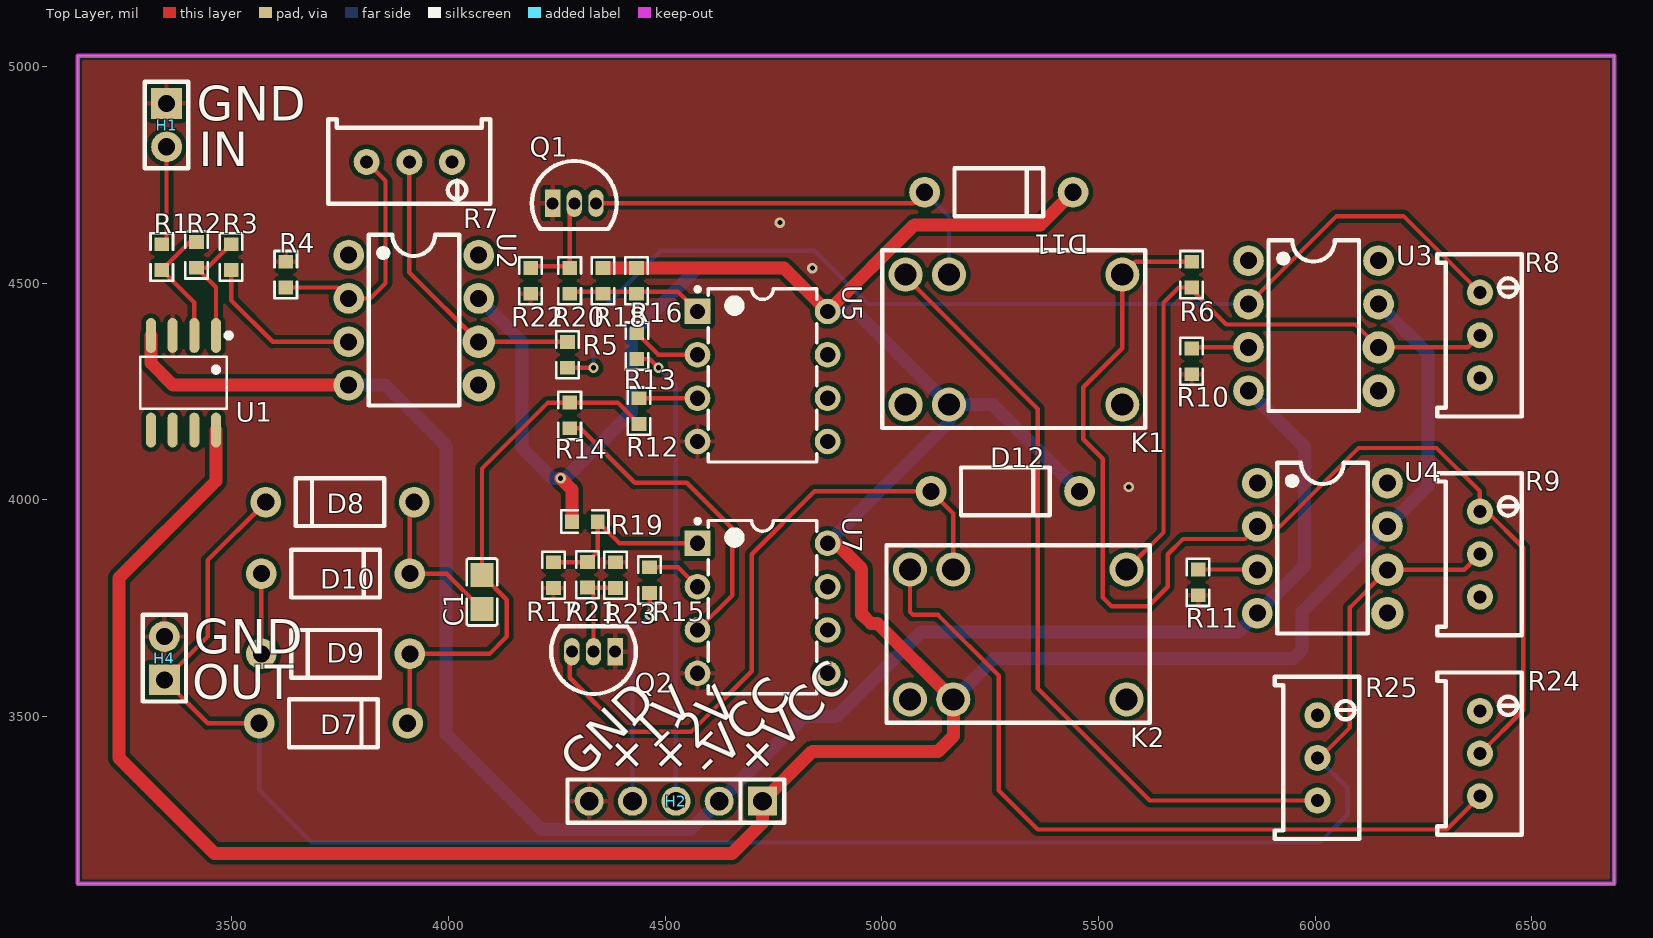
[diagram p0: Top Layer view]
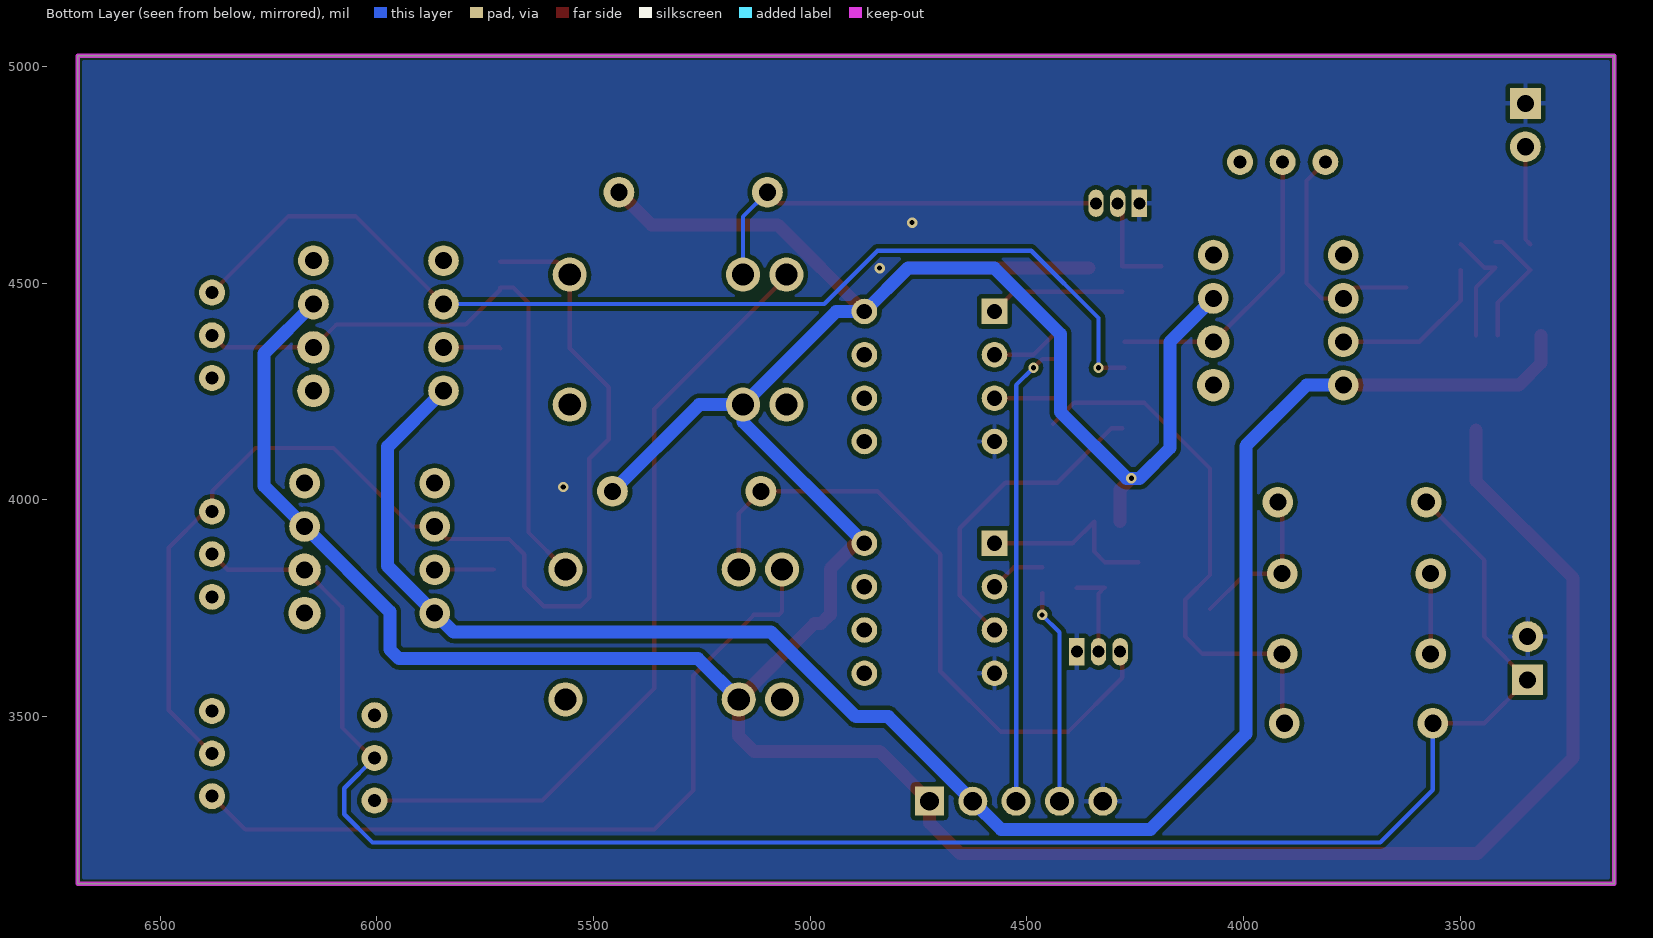
[diagram p1: Bottom Layer view, seen from below]
# Altium PCB MISC51828.pcbdoc
Units mil, origin at the board's own origin, x right, y up, seen from the top; angles counter-clockwise.
Board outline 3545 x 1910 mil, 2 copper layers (Top Layer, Bottom Layer), stack 62.206 mil thick; 45 components, 32 nets, 144 pads, 7 vias.

## Layer stack, top to bottom
Top Solder Mask Layer: solder mask 0.394, Dk 3.3
Top Layer: signal copper 1.379
Dielectric1: surface 59.449, FR4, Dk 4.5
Bottom Layer: signal copper 1.378
Bottom Solder Mask Layer: solder mask 0.394, Dk 3.3

## Board outline
3145,5025 3145,3115 6690,3115 6690,5025

## Design rules (kind name [scope] priority, off if disabled: settings)
BoardOutlineClearance copperThickness2oz_1 [All] p2 off: genericclearance=7.99 ignorepadtopadclearanceinfootprint=FALSE except(0: Arc-SplitContinuation Track-SplitContinuation SMDPad-SplitContinuation THPad-SplitContinuation Via-SplitContinuation Fill-SplitContinuation Region-SplitContinuation Poly-SplitContinuation Text-SplitContinuation Hole-SplitContinuation; 5.98: Arc-CutoutEdge Track-CutoutEdge SMDPad-CutoutEdge THPad-CutoutEdge Via-CutoutEdge Text-CutoutEdge; 6.9: Hole-OutlineEdge Hole-CutoutEdge; 10: Poly-OutlineEdge Poly-CutoutEdge; 11.81: Arc-OutlineEdge Track-OutlineEdge SMDPad-OutlineEdge THPad-OutlineEdge Via-OutlineEdge Fill-OutlineEdge Region-OutlineEdge Text-OutlineEdge Fill-CutoutEdge Region-CutoutEdge)
BoardOutlineClearance Plane_innerPlane_1 [All] p4 off: genericclearance=4.02 ignorepadtopadclearanceinfootprint=FALSE except(0: Arc-SplitContinuation Track-SplitContinuation SMDPad-SplitContinuation THPad-SplitContinuation Via-SplitContinuation Fill-SplitContinuation Region-SplitContinuation Poly-SplitContinuation Text-SplitContinuation Hole-SplitContinuation; 5.98: Arc-CutoutEdge Track-CutoutEdge SMDPad-CutoutEdge THPad-CutoutEdge Via-CutoutEdge Text-CutoutEdge; 6.9: Hole-OutlineEdge Hole-CutoutEdge; 10: Poly-OutlineEdge Poly-CutoutEdge; 11.81: Arc-OutlineEdge Track-OutlineEdge SMDPad-OutlineEdge THPad-OutlineEdge Via-OutlineEdge Fill-OutlineEdge Region-OutlineEdge Text-OutlineEdge Fill-CutoutEdge Region-CutoutEdge)
BoardOutlineClearance Copper_copperRegion_1 [All] p6 off: genericclearance=4.02 ignorepadtopadclearanceinfootprint=FALSE except(0: Arc-SplitContinuation Track-SplitContinuation SMDPad-SplitContinuation THPad-SplitContinuation Via-SplitContinuation Fill-SplitContinuation Region-SplitContinuation Poly-SplitContinuation Text-SplitContinuation Hole-SplitContinuation; 5.98: Arc-CutoutEdge Track-CutoutEdge SMDPad-CutoutEdge THPad-CutoutEdge Via-CutoutEdge Text-CutoutEdge; 6.9: Hole-OutlineEdge Hole-CutoutEdge; 10: Poly-OutlineEdge Poly-CutoutEdge; 11.81: Arc-OutlineEdge Track-OutlineEdge SMDPad-OutlineEdge THPad-OutlineEdge Via-OutlineEdge Fill-OutlineEdge Region-OutlineEdge Text-OutlineEdge Fill-CutoutEdge Region-CutoutEdge)
BoardOutlineClearance copperThickness1oz_1 [All] p8: genericclearance=4.02 ignorepadtopadclearanceinfootprint=FALSE except(0: Arc-SplitContinuation Track-SplitContinuation SMDPad-SplitContinuation THPad-SplitContinuation Via-SplitContinuation Fill-SplitContinuation Region-SplitContinuation Poly-SplitContinuation Text-SplitContinuation Hole-SplitContinuation; 5.98: Arc-CutoutEdge Track-CutoutEdge SMDPad-CutoutEdge THPad-CutoutEdge Via-CutoutEdge Text-CutoutEdge; 6.9: Hole-OutlineEdge Hole-CutoutEdge; 10: Poly-OutlineEdge Poly-CutoutEdge; 11.81: Arc-OutlineEdge Track-OutlineEdge SMDPad-OutlineEdge THPad-OutlineEdge Via-OutlineEdge Fill-OutlineEdge Region-OutlineEdge Text-OutlineEdge Fill-CutoutEdge Region-CutoutEdge)
Clearance copperThickness2oz [All] p1 off: gap=7.99 ignorepadtopadclearanceinfootprint=FALSE except(5.98: SMDPad-Track SMDPad-SMDPad THPad-Track SMDPad-THPad THPad-THPad Track-Via SMDPad-Via THPad-Via Via-Via Fill-SMDPad Region-SMDPad Fill-THPad Region-THPad Fill-Via Region-Via Fill-Fill Fill-Region Region-Region Arc-Track Arc-SMDPad Arc-THPad Arc-Via Fill-Arc Region-Arc Arc-Arc Text-Track SMDPad-Text Text-THPad Text-Via Fill-Text Region-Text Arc-Text Text-Text; 6.9: Hole-Track Hole-SMDPad Hole-THPad Hole-Via Fill-Hole Region-Hole Hole-Arc Hole-Text; 10: Poly-Track Poly-SMDPad Poly-THPad Poly-Via Poly-Fill Poly-Region Poly-Poly Poly-Arc Poly-Text Poly-Hole; 11.81: Fill-Track Region-Track)
Clearance Plane_innerPlane [All] p3 off: gap=4.02 ignorepadtopadclearanceinfootprint=FALSE except(5.98: SMDPad-Track SMDPad-SMDPad THPad-Track SMDPad-THPad THPad-THPad Track-Via SMDPad-Via THPad-Via Via-Via Fill-SMDPad Region-SMDPad Fill-THPad Region-THPad Fill-Via Region-Via Fill-Fill Fill-Region Region-Region Arc-Track Arc-SMDPad Arc-THPad Arc-Via Fill-Arc Region-Arc Arc-Arc Text-Track SMDPad-Text Text-THPad Text-Via Fill-Text Region-Text Arc-Text Text-Text; 6.9: Hole-Track Hole-SMDPad Hole-THPad Hole-Via Fill-Hole Region-Hole Hole-Arc Hole-Text; 10: Poly-Track Poly-SMDPad Poly-THPad Poly-Via Poly-Fill Poly-Region Poly-Poly Poly-Arc Poly-Text Poly-Hole; 11.81: Fill-Track Region-Track)
Clearance Copper_copperRegion [All] p5 off: gap=4.02 ignorepadtopadclearanceinfootprint=FALSE except(5.98: SMDPad-Track SMDPad-SMDPad THPad-Track SMDPad-THPad THPad-THPad Track-Via SMDPad-Via THPad-Via Via-Via Fill-SMDPad Region-SMDPad Fill-THPad Region-THPad Fill-Via Region-Via Fill-Fill Fill-Region Region-Region Arc-Track Arc-SMDPad Arc-THPad Arc-Via Fill-Arc Region-Arc Arc-Arc Text-Track SMDPad-Text Text-THPad Text-Via Fill-Text Region-Text Arc-Text Text-Text; 6.9: Hole-Track Hole-SMDPad Hole-THPad Hole-Via Fill-Hole Region-Hole Hole-Arc Hole-Text; 10: Poly-Track Poly-SMDPad Poly-THPad Poly-Via Poly-Fill Poly-Region Poly-Poly Poly-Arc Poly-Text Poly-Hole; 11.81: Fill-Track Region-Track)
Clearance copperThickness1oz [All] p7: gap=4.02 ignorepadtopadclearanceinfootprint=FALSE except(5.98: SMDPad-Track SMDPad-SMDPad THPad-Track SMDPad-THPad THPad-THPad Track-Via SMDPad-Via THPad-Via Via-Via Fill-SMDPad Region-SMDPad Fill-THPad Region-THPad Fill-Via Region-Via Fill-Fill Fill-Region Region-Region Arc-Track Arc-SMDPad Arc-THPad Arc-Via Fill-Arc Region-Arc Arc-Arc Text-Track SMDPad-Text Text-THPad Text-Via Fill-Text Region-Text Arc-Text Text-Text; 6.9: Hole-Track Hole-SMDPad Hole-THPad Hole-Via Fill-Hole Region-Hole Hole-Arc Hole-Text; 10: Poly-Track Poly-SMDPad Poly-THPad Poly-Via Poly-Fill Poly-Region Poly-Poly Poly-Arc Poly-Text Poly-Hole; 11.81: Fill-Track Region-Track)
DiffPairsRouting differentialPair [All] p1: maxlimit=6 minlimit=6 mostfreqgap=6 toplayer_minwidth=5 toplayer_prefwidth=10 toplayer_maxwidth=100 toplayer_mingap=6 toplayer_prefgap=6 toplayer_maxgap=6 bottomlayer_minwidth=5 bottomlayer_prefwidth=10 bottomlayer_maxwidth=100 bottomlayer_mingap=6 bottomlayer_prefgap=6 bottomlayer_maxgap=6 maxuncoupledlength=10
HoleToHoleClearance otherClearance [All] p1: gap=11.81 allowstackedmicrovias=TRUE
Length netLength [All] p1: minlimit=0 maxlimit=0
PasteMaskExpansion pasteMaskExpansion [All] p1: expansion=0
PlaneConnect innerPlane [All] p1: planeconnectstyle=Relief reliefexpansion=20 reliefentries=4 reliefconductorwidth=10 reliefairgap=10
PolygonConnect copperRegion [All] p1: connectstyle=Relief reliefconductorwidth=10 reliefentries=4 polygonreliefangle="90 Angle" airgapwidth=10 via.connectstyle=Relief via.reliefconductorwidth=10 via.reliefentries=4 via.polygonreliefangle="90 Angle" via.airgapwidth=10
RoutingVias viaSize [All] p1: holewidth=12.01 width=24.02 viastyle="Through Hole" minholewidth=11.81 minwidth=19.68 maxholewidth=248.03 maxwidth=393.7
SolderMaskExpansion solderMaskExpansion [IsVia] p1: expansion=-1000 istentingtop=TRUE
SolderMaskExpansion solderMaskExpansion [All] p2: expansion=2 istentingtop=FALSE
Width copperThickness2oz_2 [All] p1 off: maxlimit=100 minlimit=8 preferedwidth=10
Width copperThickness1oz_2 [All] p2: maxlimit=100 minlimit=5 preferedwidth=10

## Components (designator, comment, footprint, x,y, rotation, side; value= is the part's Value field where it differs from the comment)
C1 "22uf" C0805 4077.75,3787.74 r90 top
D7 "1N4001-TP" DO-41_BD2.4-L4.7-P8.70-D0.9-RD 3735,3485 r180 top
D8 "1N4001-TP" DO-41_BD2.4-L4.7-P8.70-D0.9-RD 3750,3995 r0 top
D9 "1N4001-TP" DO-41_BD2.4-L4.7-P8.70-D0.9-RD 3740,3645 r0 top
D10 "1N4001-TP" DO-41_BD2.4-L4.7-P8.70-D0.9-RD 3740,3830 r180 top
D11 "1N4148" DO-41_BD2.4-L4.7-P8.70-D0.9-RD 5270,4710 r180 top
D12 "1N4148" DO-41_BD2.4-L4.7-P8.70-D0.9-RD 5285,4020 r180 top
H1 "" HDR-TH_2P-P2.54-V-M-1 3350,4865 r270 top
H2 "" HDR-TH_5P-P2.54-V-M 4525,3305 r180 top
H4 "" HDR-TH_2P-P2.54-V-M-1 3345,3635 r90 top
K1 "HRS1H-S-DC5V" RELAY-TH_HRS1H-S-DC3V 5305,4370 r180 top
K2 "HRS1H-S-DC5V" RELAY-TH_HRS1H-S-DC3V 5315,3690 r180 top
Q1 "2N3904" TO-92-3_L4.9-W3.7-P1.27-L 4290.66,4684.46 r0 top
Q2 "2N3904" TO-92-3_L4.9-W3.7-P1.27-L 4335,3650 r180 top
R1 "10K" R0603 3338.93,4560.48 r270 top
R2 "10K" R0603 3418.93,4565.48 r270 top
R3 "1K" R0603 3498.93,4560.48 r270 top
R4 "1K" R0603 3625,4520 r270 top
R5 "1K" R0603 4275,4335 r270 top
R6 "1K" R0603 5715,4520 r90 top
R7 "10kΩ" R_3296 3910,4775 r180 top
R8 "10kΩ" R_3296 6385,4380 r270 top
R9 "10kΩ" R_3296 6385,3875 r270 top
R10 "1K" R0603 5715,4320 r90 top
R11 "1K" R0603 5730,3810 r90 top
R12 "1K" R0603 4440,4205 r90 top
R13 "1K" R0603 4435,4355 r90 top
R14 "1K" R0603 4280,4195 r270 top
R15 "1K" R0603 4464.41,3815.13 r90 top
R16 "3K" R0603 4434.27,4505.73 r270 top
R17 "3K" R0603 4242.68,3826.47 r90 top
R18 "1K" R0603 4356.95,4505.73 r90 top
R19 "1K" R0603 4315,3950 r180 top
R20 "1K" R0603 4280,4505.73 r90 top
R21 "1K" R0603 4320.86,3827.53 r270 top
R22 "1K" R0603 4190,4505.73 r270 top
R23 "1K" R0603 4385.45,3826.49 r90 top
R24 "100kΩ" R_3296 6385,3415 r270 top
R25 "100kΩ" R_3296 6010,3405 r270 top
U1 "LF353D" SOIC-8_L4.9-W3.9-P1.27-LS6.0-BL 3388.93,4270.48 r180 top
U2 "ADOP37AQ" PDIP-8_L9.6-W6.4-P2.54-LS7.6-BL 3920,4415 r270 top
U3 "ADOP37AQ" PDIP-8_L9.6-W6.4-P2.54-LS7.6-BL 5996.12,4402.11 r270 top
U4 "ADOP37AQ" PDIP-8_L9.6-W6.4-P2.54-LS7.6-BL 6016.61,3888.87 r270 top
U5 "LM393P" DIP-8_L10.1-W6.3-P2.54-LS7.6-BL-1 4725,4285 r270 top
U7 "LM393P" DIP-8_L10.1-W6.3-P2.54-LS7.6-BL-1 4725,3750 r270 top

## Footprints (in the part's own frame and the unit in brackets; to place one, negate y for a bottom-side part, rotate by r counter-clockwise, add the part's x,y. Pads: shape width x height; smd on the part's side, far side on the other; paste and mask are expansions set on the pad)
C0805 [mm]
  rect 1.41x1.35 smd paste-100 mask+0.051: 1(-1,0) 2(1,0)
  silkscreen extent -1.96,-0.9 1.96,0.9
DIP-8_L10.1-W6.3-P2.54-LS7.6-BL-1 [mm]
  rect 1.5x1.5 hole 0.9: 1(-3.81,-3.81)
  round 1.5 hole 0.9: 2(-1.27,-3.81) 3(1.27,-3.81) 4(3.81,-3.81) 5(3.81,3.81) 6(1.27,3.81) 7(-1.27,3.81) 8(-3.81,3.81)
  silkscreen extent -5.23,-3.93 5.01,3.18
DO-41_BD2.4-L4.7-P8.70-D0.9-RD [mm]
  round 1.8 hole 1: 1(-4.35,0) 2(4.35,0)
  silkscreen extent -2.6,-1.4 2.6,1.4
HDR-TH_2P-P2.54-V-M-1 [mm]
  rect 1.8x1.8 hole 1: 1(-1.27,0)
  round 1.8 hole 1: 2(1.27,0)
  silkscreen extent -2.54,-1.27 2.54,1.27
HDR-TH_5P-P2.54-V-M [mm]
  rect 1.7x1.7 hole 1.1: 1(-5.08,0)
  round 1.7 hole 1.1: 2(-2.54,0) 3(0,0) 4(2.54,0) 5(5.08,0)
  silkscreen extent -6.35,-1.27 6.35,1.27
PDIP-8_L9.6-W6.4-P2.54-LS7.6-BL [mm]
  round 1.8 hole 1: 1(-3.81,-3.81) 2(-1.27,-3.81) 3(1.27,-3.81) 4(3.81,-3.81) 7(-1.27,3.81) 8(-3.81,3.81)
  round 1.905 hole 1: 5(3.81,3.81) 6(1.27,3.81)
  silkscreen extent -5,-2.64 5,2.67
R0603 [mil]
  rect 31.75x34.02 smd paste-3937.01 mask+2: 1(-29.66,0) 2(29.66,0)
  silkscreen extent -55,-26 55,26
R_3296 [mil]
  round 60 hole 30 paste+0 mask+2: 1(-98.4,-5) 2(0,-5) 3(98.4,-5)
  silkscreen extent -187,-103 187,92
RELAY-TH_HRS1H-S-DC3V [mm]
  round 2 hole 1.3: 1(-6.35,-3.81) 2(3.81,-3.81) 3(6.35,-3.81) 4(6.35,3.81) 5(3.81,3.81) 6(-6.35,3.81)
  silkscreen extent -7.7,-5.23 7.72,5.18
SOIC-8_L4.9-W3.9-P1.27-LS6.0-BL [mm]
  oval 0.588x2.045 smd: 1(-1.905,-2.772) 2(-0.635,-2.772) 3(0.635,-2.772) 4(1.905,-2.772) 5(1.905,2.772) 6(0.635,2.772) 7(-0.635,2.772) 8(-1.905,2.772)
  silkscreen extent -2.8,-2.92 2.53,1.52
TO-92-3_L4.9-W3.7-P1.27-L [mm]
  rect 0.9x1.6 hole 0.7: 1(-1.27,0)
  oval 0.9x1.6 hole 0.7: 2(0,0) 3(1.27,0)
  silkscreen extent -2.48,-1.5 2.48,2.48

## Via types
v1: diameter 24.02, hole 12, Top Layer to Bottom Layer, 5 vias
v2: diameter 24, hole 12, Top Layer to Bottom Layer, 2 vias

## Nets (pads, with @x,y where several pads share a name; then routed paths per layer and width w, separated by ;. In a path a pad name is that pad's centre, name@x,y a point inside that pad or via, vN(x,y) a via of type N, cw(c..) or ccw(c..) an arc to the next point about the centre after c; other vN are vias at no path point)
1V: H2.4 R15.1 | length 497.3
  Top Layer w10: R15.1 4465,3784.88 v2(4465,3735)
  Bottom Layer w10: H2.4 4425,3695 v2(4465,3735)
2V: H2.3 R13.1 | length 1075
  Top Layer w10: R13.1 4464.66,4325.34 v2(4485,4305)
  Bottom Layer w10: v2(4485,4305) 4525,4265 H2.3
$1N134: H1.2 R1.1 | length 229.4
  Top Layer w10: R1.1 3350,4601.21 H1.2
$1N649: R1.2 R2.1 U1.2 | length 288.9
  Top Layer w10: U1.2 3413.93,4455.82 R1.2 3403.25,4595.14 R2.1
$1N688: R2.2 R3.1 U1.1 | length 277.3
  Top Layer w10: U1.1 3463.93,4490.82 R2.2 3444.61,4535.82 R3.1
$1N965: R3.2 U2.3 | length 380.6
  Top Layer w10: R3.2 3498.93,4461.07 3595,4365 U2.3
$1N1004: R4.2 R7.3 U2.2 | length 553
  Top Layer w10: R4.2 3744.66,4490.34 U2.2 3820,4465 3855,4500 3855,4736.6 R7.3
$1N1351: R5.1 R7.2 U2.6 | length 686.4
  Top Layer w10: R7.2 3910,4525 U2.6 4274.66,4365 R5.1
$1N1453: R5.2 R8.1 U3.2 | length 2492.4
  Top Layer w10: R5.2 4275.34,4305 v1(4335,4305) ; U3.2 6049.01,4655 6203.4,4655 R8.1
  Bottom Layer w10: v1(4335,4305) 4335,4420 4490,4575 4845,4575 4967.89,4452.11 U3.2
$1N1523: R10.2 U3.3 | length 132.1
  Top Layer w10: R10.2 5717.45,4352.11 U3.3
$1N1566: K2.1 R6.1 R8.2 U3.6 | length 1466.8
  Top Layer w10: K2.1 5650,3925 5650,4455 5685.34,4490.34 R6.1 5715,4485 5795,4405 6093.23,4405 U3.6 6352.11,4352.11 R8.2
$1N1670: K1.1 R6.2 R9.1 R24.2 U4.2 | length 2785.6
  Top Layer w10: R6.2 5584.66,4549.66 K1.1 5555,4350 5465,4260 5465,4140 5510,4095 5510,3775 5530,3755 5615,3755 5660,3800 5660,3875 5695,3910 5837.74,3910 U4.2 5918.87,3938.87 6100,4120 6280,4120 6380,4020 R9.1 6396.6,3973.4 6480,3890 6480,3515 R24.2
$1N1716: R11.2 U4.3 | length 136.9
  Top Layer w10: R11.2 5865.82,3839.66 U4.3
$1N1759: D7.2 D8.1 H4.1 R9.2 R25.2 U4.6 | length 4400.2
  Top Layer w10: D7.2 3445,3485 H4.1 3445,3685 3445,3861.26 D8.1 ; R25.2 6010,3405 6080,3475 6080,3752.26 U4.6 6343.87,3838.87 R9.2
  Bottom Layer w10: D7.2 3563.74,3331.26 3685,3210 6010,3210 6075,3275 6075,3335 R25.2
$1N2598: K1.3 R25.3 | length 1833.4
  Top Layer w10: K1.3 5055,4515 5360,4210 5360,3565 5618.4,3306.6 R25.3
$1N2700: D11.2 K1.2 Q1.3 | length 982
  Top Layer w10: Q1.3 5073.2,4684.46 D11.2
  Bottom Layer w10: D11.2 5155,4653.74 K1.2
$1N2816: K2.3 R24.3 | length 1807.9
  Top Layer w10: K2.3 5065,3742.07 5072.07,3735 5130,3735 5270,3595 5270,3330 5360,3240 6303.4,3240 R24.3
$1N2866: D12.2 K2.2 Q2.3 | length 1536.9
  Top Layer w10: Q2.3 4280,3645 4280,3590 4405,3465 4560,3465 4700,3605 4700,3875 4845,4020 D12.2 5165,3968.74 K2.2
$1N3061: Q1.2 R20.2 R22.1 | length 239.2
  Top Layer w10: R22.1@4190,4539.66 4280,4539.66 4280,4673.8 Q1.2
$1N3114: R16.2 R18.1 R20.1 U5.1 | length 313.8
  Top Layer w10: R20.1@4280,4480.34 4529.66,4480.34 U5.1
$1N3909: R12.2 U5.3 | length 135.1
  Top Layer w10: R12.2 4574.66,4234.66 U5.3
$1N3935: R13.2 U5.2 | length 160.6
  Top Layer w10: R13.2 4484.66,4335 U5.2
$1N3964: C1.2 D7.1 D9.2 R12.1 R14.1 | length 1259.4
  Top Layer w10: D7.1 3911.26,3490 D9.2 4095,3645 4135,3685 4135,3769.86 C1.2 4077.75,4072.75 4229.66,4224.66 R14.1 4390.68,4224.66 R12.1
$1N4101: R14.2 U7.3 | length 738.5
  Top Layer w10: R14.2 4304.66,4165.34 4430,4040 4550,4040 4655,3935 4655,3780 U7.3
$1N4103: R15.2 U7.2 | length 129.1
  Top Layer w10: R15.2 4530.21,3844.79 U7.2
$1N4238: R17.2 R19.1 R21.1 U7.1 | length 432.3
  Top Layer w10: R17.2 4319.8,3856.13 R21.1 4344.66,3880.99 R19.1 4394.66,3900 U7.1
$1N4251: Q2.2 R21.2 R23.1 | length 218.8
  Top Layer w10: Q2.2 4335,3783.72 R21.2 4384.42,3797.87 R23.1
$1N4430: C1.1 D8.2 D10.1 | length 369.4
  Top Layer w10: D8.2 3911.26,3985 D10.1 3996.12,3830 C1.1
$1N4435: D9.1 D10.2 | length 185
  Top Layer w10: D9.1 D10.2
-VCC: H2.2 U1.4 U2.4 U3.4 U4.4 | length 4269.7
  Top Layer w30: U1.4 3313.93,4316.07 3365,4265 U2.4
  Bottom Layer w30: U2.4 3855,4265 3995,4125 3995,3460 4215,3240 4560,3240 H2.2 4820,3500 4895,3500 5090,3695 5822.74,3695 U4.4 5975,3847.26 5975,4123.23 U3.4
GND: H1.1 H2.5 H4.2 Q1.1 Q2.1 R4.1 R10.1 R11.1 R17.1 R22.2 R23.2 U1.3 U5.4 U7.4
  other v1: 5570,4030 4840,4535 4765,4640
VCC: D11.1 D12.1 H2.1 K1.5 K2.5 R16.1 R18.2 R19.2 U1.8 U2.7 U3.7 U4.7 U5.8 U7.8 | length 9417
  Top Layer w30: U1.8 3463.93,4043.93 3240,3820 3240,3405 3460,3185 4655,3185 4725,3255 H2.1 4840,3420 5130,3420 5165,3455 K2.5 4990,3715 4975,3715 4953.79,3736.21 4953.79,3841.21 4895,3900 U7.8 ; v1(4259.15,4050) 4285.34,4023.81 R19.2 ; R18.2 R16.1 4774.61,4535.39 U5.8 5075,4635 5366.26,4635 D11.1
  Bottom Layer w30: U2.7 4170,4365 4170,4120 4240,4050 4270,4050 4422.5,4202.5 4422.5,4382.5 4575,4535 4775,4535 U5.8 4940,4435 K1.5 ; U7.8 5155,4180 K1.5 ; K2.5 5258.79,3633.79 5948.79,3633.79 5970,3655 5970,3742.26 U4.7 6260,4032.26 6260,4338.23 U3.7 ; D12.1 5256.26,4220 K1.5
pads on no net: K1.4 K1.6 K2.4 K2.6 R7.1 R8.3 R9.3 R24.1 R25.1 U1.5 U1.6 U1.7 U2.1 U2.5 U2.8 U3.1 U3.5 U3.8 U4.1 U4.5 U4.8 U5.5 U5.6 U5.7 U7.5 U7.6 U7.7

## Polygon pours and split planes (outlines as drawn)
GND on Top Layer (solid, remove dead copper, pour order 0): 3000,5090 3000,3000 6860,3000 6860,5090
GND on Bottom Layer (solid, remove dead copper, pour order 2): 3120,5075 3120,3035 6835,3035 6835,5075

## Keep-outs
Board Outline Layer:
  the board outline again, w10

## Silkscreen, mask and mechanical layers (free items; w line width, h text height)
Top Silkscreen Layer:
  text "GND" at 3420,4875 h80
  text "IN" at 3423.8,4770 h80
  text "GND" at 3412.34,3645 h80
  text "OUT" at 3408.8,3540 h80
  text "GND" at 4305.31,3355 h80 r45
  text "+1V" at 4405.31,3355 h80 r45
  text "+2V" at 4505.31,3355 h80 r45
  text "-VCC" at 4605.31,3355 h80 r45
  text "+VCC" at 4705.31,3355 h80 r45